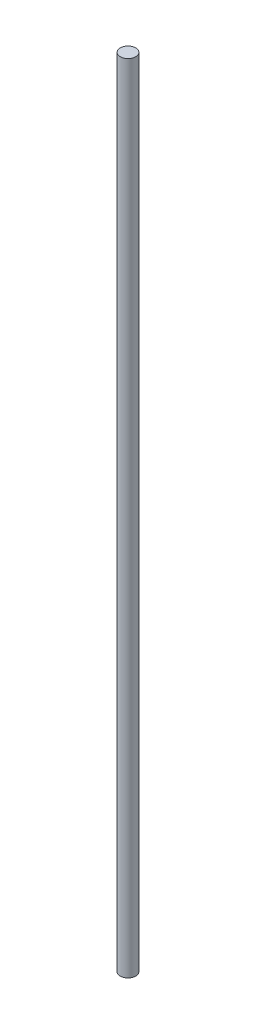
SolidWorks part; units mm, degrees
material "ABS"
ref_plane "前视基准面" through (0, 0, 0) normal (0, 0, 1) x (1, 0, 0)
ref_plane "上视基准面" through (0, 0, 0) normal (0, 1, 0) x (1, 0, 0)
ref_plane "右视基准面" through (0, 0, 0) normal (1, 0, 0) x (0, 0, -1)
sketch "草图2" plane through (0, 0, 0) normal (0, 1, 0) x (1, 0, 0)
  circle A0 centre (0, 0) radius 1.5
  dimension "D1" = 3
extrude "凸台-拉伸1" add sketch "草图2" along normal blind 155
